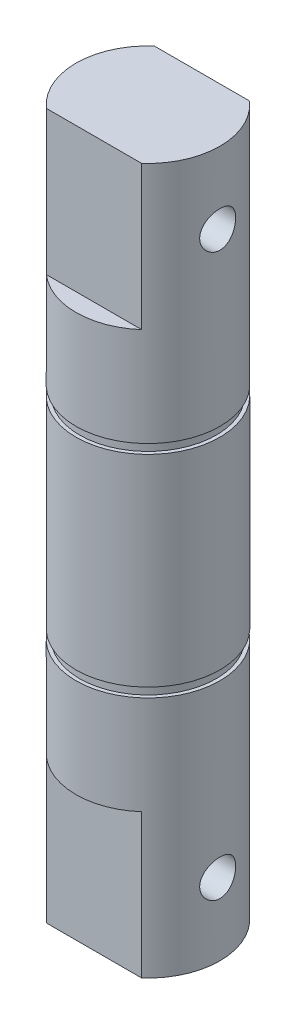
from build123d import *

# Parameters (mm, degrees)
SKETCH_1_R               = 10
EXTRUDE_1_DEPTH          = 98
CUT_EXTRUDE_1_DEPTH      = 10
CUT_EXTRUDE_1_DEPTH_BACK = 10
SKETCH_2_W               = 2.5
SKETCH_2_H               = 20
HOLE_WIZARD_M6_1_D       = 5
SKETCH_5_W               = 0.5
SKETCH_5_H               = 1.3


with BuildPart() as part:
    # 草图1 → 凸台-拉伸1 (new body)
    with BuildSketch(Plane(origin=(0, 0, 0), x_dir=(1, 0, 0), z_dir=(0, 1, 0))):
        with Locations(Location((0, 0, 0), (0, 0, 270))):
            Circle(SKETCH_1_R)
    extrude(amount=EXTRUDE_1_DEPTH)

    # 草图2 → 切除-拉伸1 (cut, two sides: drawn at the far end of the back side and taken through both)
    with BuildSketch(Plane(origin=(0, 0, 0), x_dir=(0, 0, -1), z_dir=(1, 0, 0)).offset(-CUT_EXTRUDE_1_DEPTH_BACK)):
        with Locations((8.75, 88)):
            Rectangle(SKETCH_2_W, SKETCH_2_H)
        with Locations((-8.75, 88)):
            Rectangle(SKETCH_2_W, SKETCH_2_H)
        with Locations((-8.75, 10)):
            Rectangle(SKETCH_2_W, SKETCH_2_H)
        with Locations((8.75, 10)):
            Rectangle(SKETCH_2_W, SKETCH_2_H)
    extrude(amount=CUT_EXTRUDE_1_DEPTH + CUT_EXTRUDE_1_DEPTH_BACK, mode=Mode.SUBTRACT)

    # M6 螺纹孔1 (through all)
    with Locations(Plane(origin=(10, 0, 0), x_dir=(0, 0, -1), z_dir=(1, 0, 0))):
        with Locations((0, 88), (0, 10)):
            Hole(HOLE_WIZARD_M6_1_D / 2)

    # 草图5 → 切除-旋转1 (revolve, cut)
    with BuildSketch(Plane.XY, mode=Mode.PRIVATE) as cut_revolve_1_sk:
        with Locations((-9.75, 63.65)):
            Rectangle(SKETCH_5_W, SKETCH_5_H)
        with Locations((-9.75, 34.35)):
            Rectangle(SKETCH_5_W, SKETCH_5_H)
    revolve(cut_revolve_1_sk.sketch.rotate(Axis((0, 98, 0), (0, -1, 0)), 270), axis=Axis((0, 98, 0), (0, -1, 0)), mode=Mode.SUBTRACT)


solid = part.part
